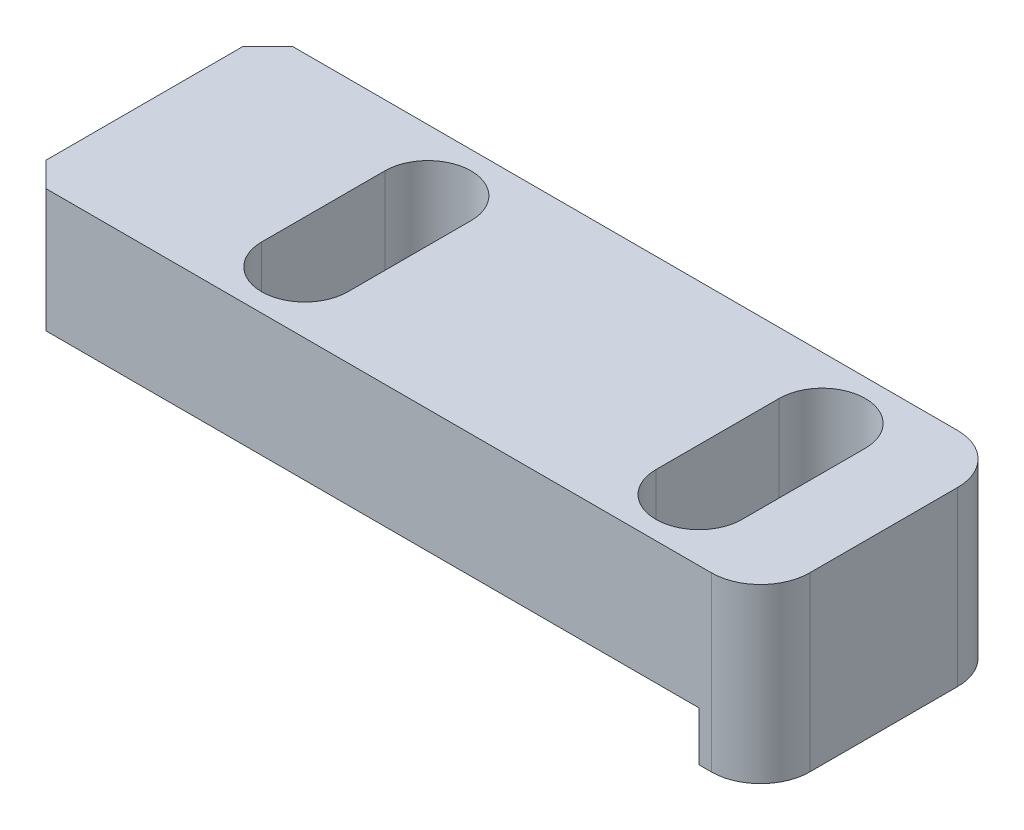
SolidWorks part; units mm, degrees
ref_plane "Front Plane" through (0, 0, 0) normal (0, 0, 1) x (1, 0, 0)
ref_plane "Top Plane" through (0, 0, 0) normal (0, 1, 0) x (1, 0, 0)
ref_plane "Right Plane" through (0, 0, 0) normal (1, 0, 0) x (0, 0, -1)
sketch "Sketch1" plane through (0, 0, 0) normal (0, 0, 1) x (1, 0, 0)
  line L1 (0, 0) -> (-30, 0)
  line L2 (0, 0) -> (0, -7)
  line L3 (0, -7) -> (-2.5, -7)
  line L4 (-30, 0) -> (-30, -5)
  line L7 (-30, -5) -> (-2.5, -5)
  line L8 (-2.5, -7) -> (-2.5, -5)
  dimension "D1" = 5
  dimension "D2" = 2.5
  dimension "D3" = 30
  dimension "D4" = 7
extrude "Boss-Extrude1" add sketch "Sketch1" along normal mid plane 10
sketch "Sketch2" plane through (0, -5, 0) normal (0, -1, 0) x (1, 0, 0)
  line L0 (-21, 2.5) -> (-21, -2.5) construction
  line L1 (-19.25, 2.5) -> (-19.25, -2.5)
  line L2 (-22.75, 2.5) -> (-22.75, -2.5)
  line L3 (-5, 2.5) -> (-5, -2.5) construction
  line L4 (-3.25, 2.5) -> (-3.25, -2.5)
  line L5 (-6.75, 2.5) -> (-6.75, -2.5)
  line L6 (0, 0) -> (-30, 0) construction
  line L7 (0, 5) -> (0, -5) construction
  line L8 (-30, 5) -> (-30, -5) construction
  arc A0 (-19.25, 2.5) -> (-22.75, 2.5) centre (-21, 2.5) ccw
  arc A1 (-22.75, -2.5) -> (-19.25, -2.5) centre (-21, -2.5) ccw
  arc A2 (-3.25, 2.5) -> (-6.75, 2.5) centre (-5, 2.5) ccw
  arc A3 (-6.75, -2.5) -> (-3.25, -2.5) centre (-5, -2.5) ccw
  point P2 (-21, 0)
  point P7 (-5, 0)
  dimension "D1" = 3.5
  dimension "D2" = 5
  dimension "D3" = 5
  dimension "D4" = 16
extrude "Cut-Extrude1" cut sketch "Sketch2" against normal through all
fillet "Fillet1" radius 2 2 edges at (0, -3.5, -5) (0, -3.5, 5)
chamfer "Chamfer1" distance 1 angle 45 2 edges at (-30, -2.5, 5) (-30, -2.5, -5)
